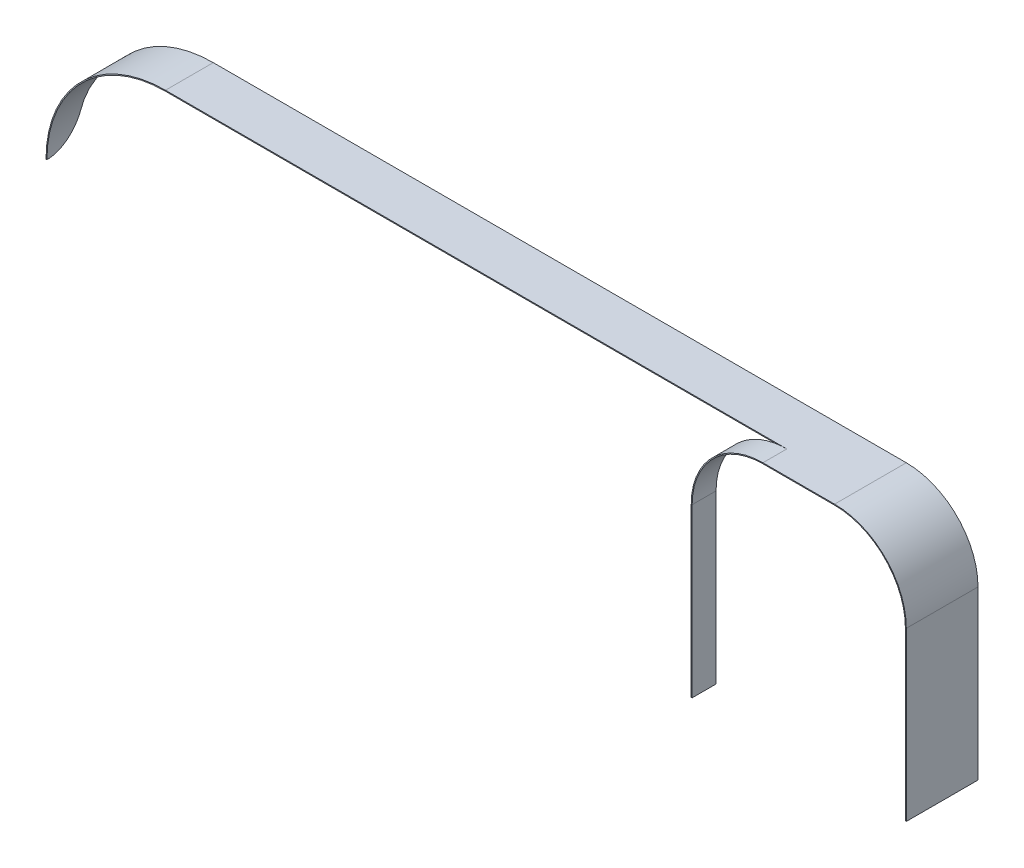
SolidWorks part; units mm, degrees
material "普通碳钢"
ref_plane "Front Plane" through (0, 0, 0) normal (0, 0, 1) x (1, 0, 0)
ref_plane "Top Plane" through (0, 0, 0) normal (0, 1, 0) x (1, 0, 0)
ref_plane "Right Plane" through (0, 0, 0) normal (1, 0, 0) x (0, 0, -1)
sketch "Sketch1" plane through (0, 0, 0) normal (0, 0, 1) x (1, 0, 0)
  line L0 (0, 254) -> (1473.2, 254)
  line L1 (1625.6, 101.6) -> (1625.6, -254)
  line L2 (-435.7297, 0) -> (474.0109, 0) construction
  line L3 (0, 445.7093) -> (0, -413.4049) construction
  line L4 (0, 252) -> (1473.2, 252)
  line L5 (1623.6, 101.6) -> (1623.6, -254)
  line L6 (-254, 0) -> (-252, 0)
  line L7 (1623.6, -254) -> (1625.6, -254)
  arc A0 (0, 254) -> (-254, 0) centre (0, 0) ccw
  arc A1 (1473.2, 254) -> (1625.6, 101.6) centre (1473.2, 101.6) cw
  arc A2 (0, 252) -> (-252, 0) centre (0, 0) ccw
  arc A3 (1473.2, 252) -> (1623.6, 101.6) centre (1473.2, 101.6) cw
  point P13 (1625.6, 254)
  dimension "D1" = 508
  dimension "D4" = 152.4
  dimension "D2" = 508
  dimension "D3" = 1625.6
  dimension "D5" = 2
extrude "Boss-Extrude1" add sketch "Sketch1" against normal blind 101.6
sketch "Sketch2" plane through (0, 0, 0) normal (0, 0, 1) x (1, 0, 0)
  line L0 (1625.6, -254) -> (1625.6, 101.6) construction
  line L1 (1473.2, 254) -> (0, 254) construction
  line L2 (1625.6, -254) -> (1625.6, 101.6)
  line L3 (1473.2, 254) -> (1320.8, 254)
  line L4 (1168.4, 101.6) -> (1168.4, -254)
  line L7 (1623.6, -254) -> (1623.6, 101.6)
  line L8 (1473.2, 252) -> (1320.8, 252)
  line L9 (1170.4, 101.6) -> (1170.4, -254)
  line L10 (1168.4, -254) -> (1170.4, -254)
  line L11 (1623.6, -254) -> (1625.6, -254)
  arc A0 (1625.6, 101.6) -> (1473.2, 254) centre (1473.2, 101.6) ccw construction
  arc A1 (1625.6, 101.6) -> (1473.2, 254) centre (1473.2, 101.6) ccw
  arc A2 (1168.4, 101.6) -> (1320.8, 254) centre (1320.8, 101.6) cw
  arc A3 (1623.6, 101.6) -> (1473.2, 252) centre (1473.2, 101.6) ccw
  arc A4 (1170.4, 101.6) -> (1320.8, 252) centre (1320.8, 101.6) cw
  dimension "D2" = 152.4
  dimension "D1" = 457.2
  dimension "D3" = 2
extrude "Boss-Extrude2" add sketch "Sketch2" along normal blind 50.8
sketch "Sketch3" plane through (0, 0, 0) normal (1, 0, 0) x (0, 0, -1)
  line L0 (101.6, 101.6) -> (101.6, -254) construction
  line L1 (101.6, 172.72) -> (101.6, 0)
  line L3 (101.6, 0) -> (0, 0)
  line L4 (0, 101.6) -> (0, -254) construction
  line L5 (63.5, 134.62) -> (63.5, 63.5)
  line L6 (101.6, 0) -> (101.6, 254) construction
  arc A0 (101.6, 172.72) -> (63.5, 134.62) centre (101.6, 134.62) ccw
  arc A1 (0, 0) -> (63.5, 63.5) centre (0, 63.5) ccw
  dimension "D1" = 38.1
  dimension "D3" = 127
  dimension "D2" = 172.72
extrude "Cut-Extrude1" cut sketch "Sketch3" against normal blind 800
